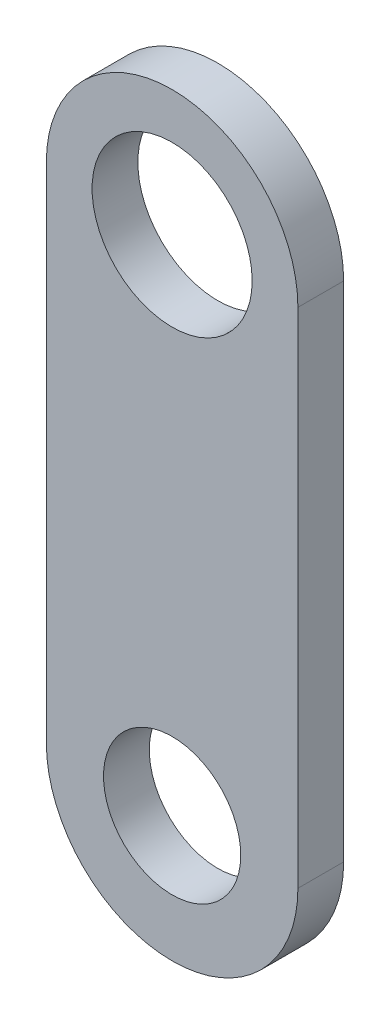
SolidWorks part; units mm, degrees
ref_plane "Front Plane" through (0, 0, 0) normal (0, 0, 1) x (1, 0, 0)
ref_plane "Top Plane" through (0, 0, 0) normal (0, 1, 0) x (1, 0, 0)
ref_plane "Right Plane" through (0, 0, 0) normal (1, 0, 0) x (0, 0, -1)
other "Configuration Table"
sketch "Sketch1" plane through (0, 0, 0) normal (0, 0, 1) x (1, 0, 0)
  line L0 (-27.5, 110) -> (-27.5, 0)
  line L1 (27.5, 110) -> (27.5, 0)
  line L2 (0, 0) -> (0, 110) construction
  circle A0 centre (0, 0) radius 15
  circle A1 centre (0, 110) radius 17.5
  arc A3 (27.5, 110) -> (-27.5, 110) centre (0, 110) ccw
  arc A4 (-27.5, 0) -> (27.5, 0) centre (0, 0) ccw
  circle A6 centre (0, 0) radius 27.5 construction
  dimension "D1" = 110
  dimension "D2" = 27.5
  dimension "D3" = 30
  dimension "D4" = 35
extrude "Boss-Extrude1" add sketch "Sketch1" along normal blind 10
